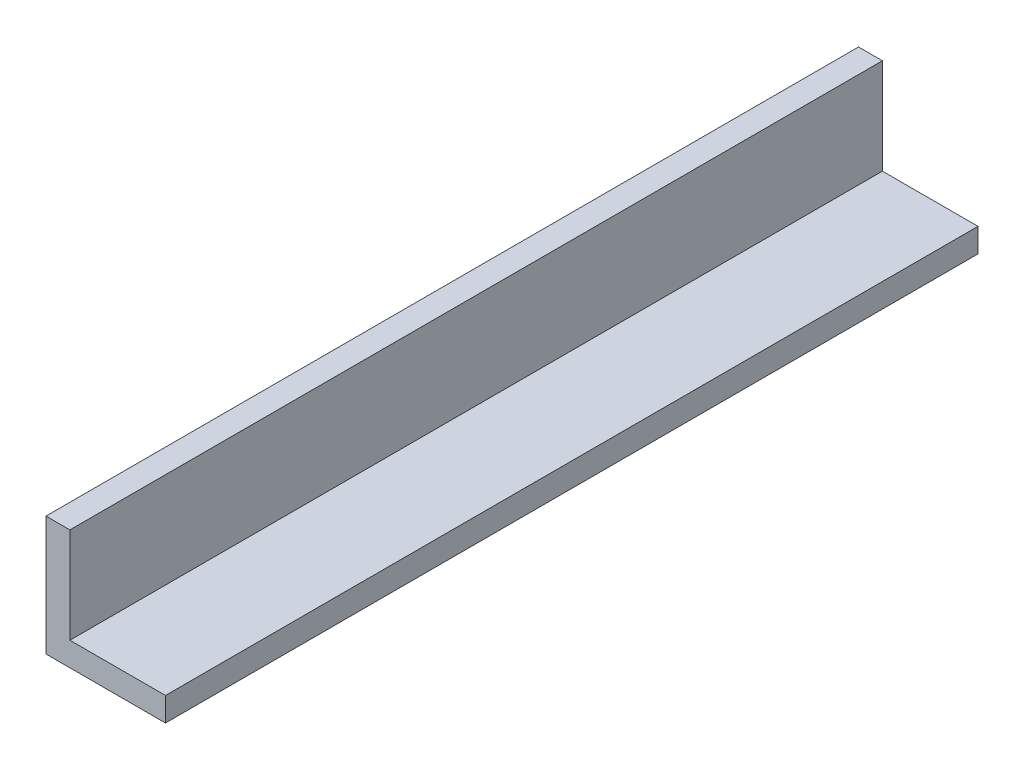
SolidWorks part; units mm, degrees
ref_plane "前视基准面" through (0, 0, 0) normal (0, 0, 1) x (1, 0, 0)
ref_plane "上视基准面" through (0, 0, 0) normal (0, 1, 0) x (1, 0, 0)
ref_plane "右视基准面" through (0, 0, 0) normal (1, 0, 0) x (0, 0, -1)
sketch "草图1" plane through (0, 0, 0) normal (0, 0, 1) x (1, 0, 0)
  line L0 (0, 0) -> (0, 25)
  line L1 (0, 25) -> (5, 25)
  line L2 (5, 25) -> (5, 5)
  line L3 (5, 5) -> (25, 5)
  line L4 (25, 5) -> (25, 0)
  line L5 (25, 0) -> (0, 0)
  dimension "D1" = 5
  dimension "D2" = 20
extrude "凸台-拉伸1" add sketch "草图1" along normal blind 170
